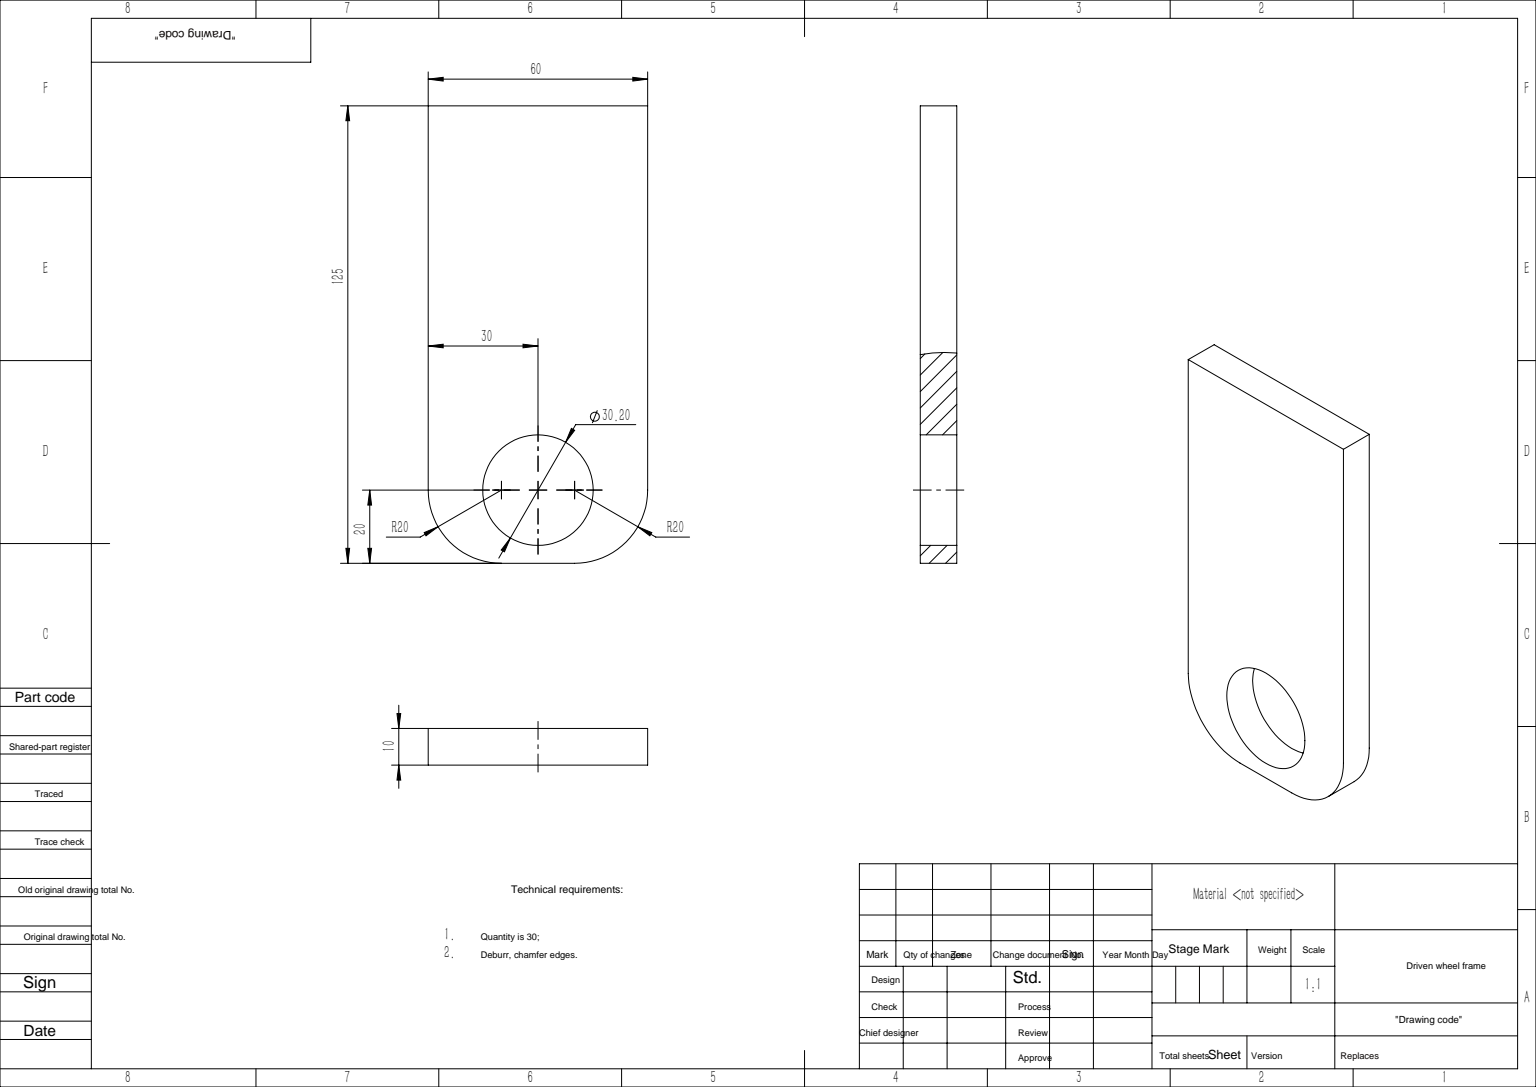
SolidWorks part; units mm, degrees
ref_plane "前视基准面" through (0, 0, 0) normal (0, 0, 1) x (1, 0, 0)
ref_plane "上视基准面" through (0, 0, 0) normal (0, 1, 0) x (1, 0, 0)
ref_plane "右视基准面" through (0, 0, 0) normal (1, 0, 0) x (0, 0, -1)
sketch "草图1" plane through (0, 0, 0) normal (0, 0, 1) x (1, 0, 0)
  line L0 (0, 0) -> (0, 100) construction
  line L1 (-30, 105) -> (30, 105)
  line L2 (-30, 105) -> (-30, -20)
  line L3 (-30, -20) -> (30, -20)
  line L4 (30, 105) -> (30, -20)
  circle A0 centre (0, 0) radius 15.1
  dimension "D1" = 30.2
  dimension "D5" = 20
  dimension "D2" = 125
  dimension "D3" = 60
  dimension "D4" = 100
extrude "凸台-拉伸1" add sketch "草图1" along normal blind 10
fillet "圆角1" radius 20 2 edges at (-30, -20, 5) (30, -20, 5)
